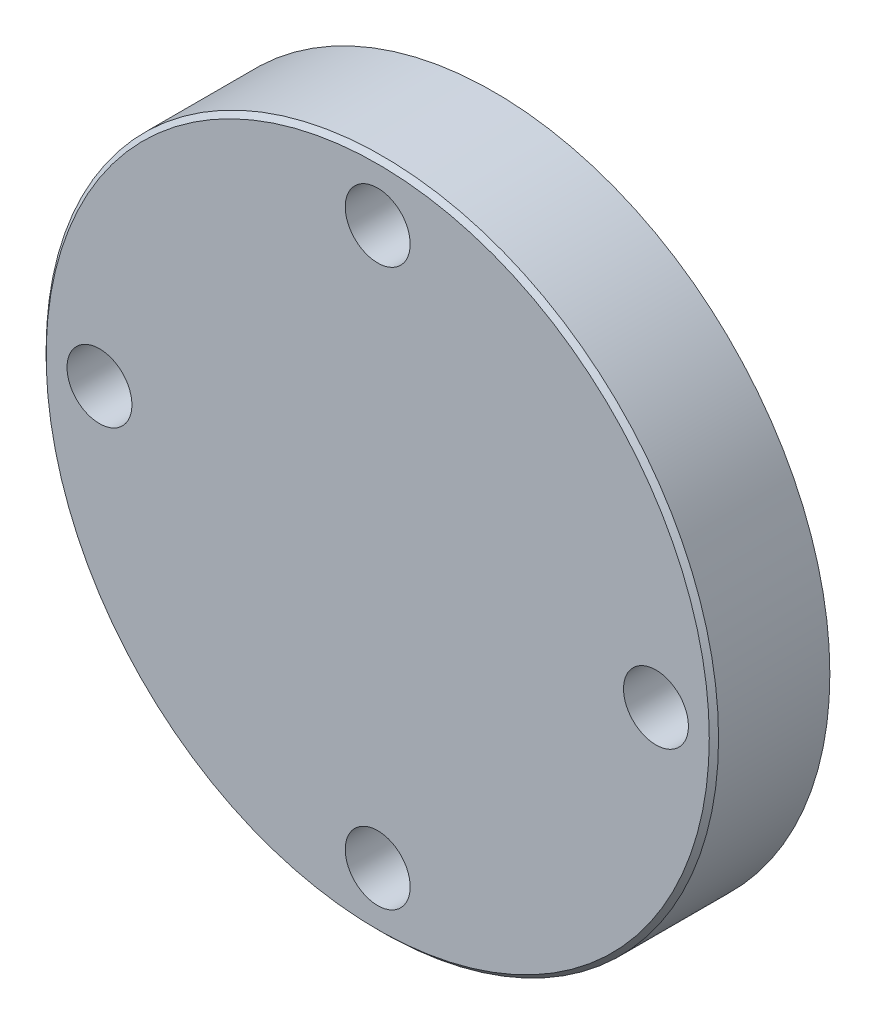
from build123d import *

# Parameters (mm, degrees)
SKETCH_1_R          = 72.5
EXTRUDE_1_DEPTH     = 25
SKETCH_2_R          = 7
CUT_EXTRUDE_1_DEPTH = 106.534354596
CUT_EXTRUDE_2_DEPTH = 15
CHAMFER_1_SIZE      = 1
CHAMFER_2_SIZE      = 1


with BuildPart() as part:
    # 草图1 → 凸台-拉伸1 (new body)
    with BuildSketch(Plane.XY):
        Circle(SKETCH_1_R)
    extrude(amount=EXTRUDE_1_DEPTH)

    # 草图2 → 切除-拉伸1 (cut, through all)
    with BuildSketch(Plane.XY.offset(25)):
        with Locations((0, 60)):
            Circle(SKETCH_2_R)
        with Locations((60, 0)):
            Circle(SKETCH_2_R)
        with Locations((0, -60)):
            Circle(SKETCH_2_R)
        with Locations((-60, 0)):
            Circle(SKETCH_2_R)
    extrude(amount=-CUT_EXTRUDE_1_DEPTH, mode=Mode.SUBTRACT)

    # 草图3 → 切除-拉伸2 (cut)
    with BuildSketch(Plane(origin=(0, 0, 0), x_dir=(-1, 0, 0), z_dir=(0, 0, -1))):
        with BuildLine():
            Line((-32.5, 36), (32.5, 36))
            ThreePointArc((32.5, 36), (48.5, 0), (32.5, -36))
            Line((32.5, -36), (-32.5, -36))
            ThreePointArc((-32.5, -36), (-48.5, 0), (-32.5, 36))
        make_face()
    extrude(amount=-CUT_EXTRUDE_2_DEPTH, mode=Mode.SUBTRACT)

    # 倒角1
    chamfer_1_edges = [part.edges().sort_by_distance(p)[0] for p in [
        (-72.5, 0, 25),
    ]]
    chamfer(chamfer_1_edges, length=CHAMFER_1_SIZE)

    # 倒角2
    chamfer_2_edges = [part.edges().sort_by_distance(p)[0] for p in [
        (48.5, 0, 0),
        (0, -36, 0),
        (-48.5, 0, 0),
        (0, 36, 0),
    ]]
    chamfer(chamfer_2_edges, length=CHAMFER_2_SIZE)


solid = part.part
